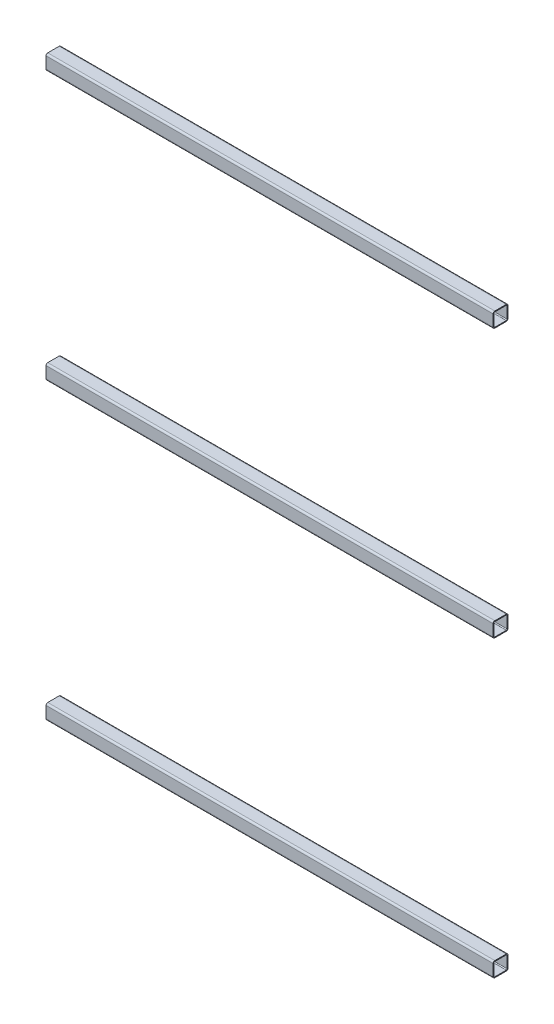
from build123d import *

# Parameters (mm, degrees)
SQUARE_TUBE_40_X_40_X_2_3_1_DEPTH   = 1200
SQUARE_TUBE_40_X_40_X_2_3_1_2_DEPTH = 1200
SQUARE_TUBE_40_X_40_X_2_3_1_3_DEPTH = 1200


with BuildPart() as part:
    # Sketch11 → Square Tube 40 X 40 X 2.3(1) (new body)
    with BuildSketch(Plane.YZ):
        with BuildLine():
            Line((-15.4, -20), (15.4, -20))
            ThreePointArc((15.4, -20), (18.652691193, -18.652691193), (20, -15.4))
            Line((20, -15.4), (20, 15.4))
            ThreePointArc((20, 15.4), (18.652691193, 18.652691193), (15.4, 20))
            Line((15.4, 20), (-15.4, 20))
            ThreePointArc((-15.4, 20), (-18.652691193, 18.652691193), (-20, 15.4))
            Line((-20, 15.4), (-20, -15.4))
            ThreePointArc((-20, -15.4), (-18.652691193, -18.652691193), (-15.4, -20))
        make_face()
        with BuildLine():
            Line((-15.4, -17.7), (15.4, -17.7))
            ThreePointArc((15.4, -17.7), (17.026345597, -17.026345597), (17.7, -15.4))
            Line((17.7, -15.4), (17.7, 15.4))
            ThreePointArc((17.7, 15.4), (17.026345597, 17.026345597), (15.4, 17.7))
            Line((15.4, 17.7), (-15.4, 17.7))
            ThreePointArc((-15.4, 17.7), (-17.026345597, 17.026345597), (-17.7, 15.4))
            Line((-17.7, 15.4), (-17.7, -15.4))
            ThreePointArc((-17.7, -15.4), (-17.026345597, -17.026345597), (-15.4, -17.7))
        make_face(mode=Mode.SUBTRACT)
    extrude(amount=SQUARE_TUBE_40_X_40_X_2_3_1_DEPTH)


with BuildPart() as body_2:
    # Sketch11 on segment 2 (carried to segment 2) → Square Tube 40 X 40 X 2.3_1 2 (new body)
    with BuildSketch(Plane(origin=(0, 1510, 0), x_dir=(0, 1, 0), z_dir=(1, 0, 0))):
        with BuildLine():
            Line((-15.4, -20), (15.4, -20))
            ThreePointArc((15.4, -20), (18.652691193, -18.652691193), (20, -15.4))
            Line((20, -15.4), (20, 15.4))
            ThreePointArc((20, 15.4), (18.652691193, 18.652691193), (15.4, 20))
            Line((15.4, 20), (-15.4, 20))
            ThreePointArc((-15.4, 20), (-18.652691193, 18.652691193), (-20, 15.4))
            Line((-20, 15.4), (-20, -15.4))
            ThreePointArc((-20, -15.4), (-18.652691193, -18.652691193), (-15.4, -20))
        make_face()
        with BuildLine():
            Line((-15.4, -17.7), (15.4, -17.7))
            ThreePointArc((15.4, -17.7), (17.026345597, -17.026345597), (17.7, -15.4))
            Line((17.7, -15.4), (17.7, 15.4))
            ThreePointArc((17.7, 15.4), (17.026345597, 17.026345597), (15.4, 17.7))
            Line((15.4, 17.7), (-15.4, 17.7))
            ThreePointArc((-15.4, 17.7), (-17.026345597, 17.026345597), (-17.7, 15.4))
            Line((-17.7, 15.4), (-17.7, -15.4))
            ThreePointArc((-17.7, -15.4), (-17.026345597, -17.026345597), (-15.4, -17.7))
        make_face(mode=Mode.SUBTRACT)
    extrude(amount=SQUARE_TUBE_40_X_40_X_2_3_1_2_DEPTH)


with BuildPart() as body_3:
    # Sketch11 on segment 3 (carried to segment 3) → Square Tube 40 X 40 X 2.3_1 3 (new body)
    with BuildSketch(Plane(origin=(0, 790, 0), x_dir=(0, 1, 0), z_dir=(1, 0, 0))):
        with BuildLine():
            Line((-15.4, -20), (15.4, -20))
            ThreePointArc((15.4, -20), (18.652691193, -18.652691193), (20, -15.4))
            Line((20, -15.4), (20, 15.4))
            ThreePointArc((20, 15.4), (18.652691193, 18.652691193), (15.4, 20))
            Line((15.4, 20), (-15.4, 20))
            ThreePointArc((-15.4, 20), (-18.652691193, 18.652691193), (-20, 15.4))
            Line((-20, 15.4), (-20, -15.4))
            ThreePointArc((-20, -15.4), (-18.652691193, -18.652691193), (-15.4, -20))
        make_face()
        with BuildLine():
            Line((-15.4, -17.7), (15.4, -17.7))
            ThreePointArc((15.4, -17.7), (17.026345597, -17.026345597), (17.7, -15.4))
            Line((17.7, -15.4), (17.7, 15.4))
            ThreePointArc((17.7, 15.4), (17.026345597, 17.026345597), (15.4, 17.7))
            Line((15.4, 17.7), (-15.4, 17.7))
            ThreePointArc((-15.4, 17.7), (-17.026345597, 17.026345597), (-17.7, 15.4))
            Line((-17.7, 15.4), (-17.7, -15.4))
            ThreePointArc((-17.7, -15.4), (-17.026345597, -17.026345597), (-15.4, -17.7))
        make_face(mode=Mode.SUBTRACT)
    extrude(amount=SQUARE_TUBE_40_X_40_X_2_3_1_3_DEPTH)


solid = Compound([part.part, body_2.part, body_3.part])
